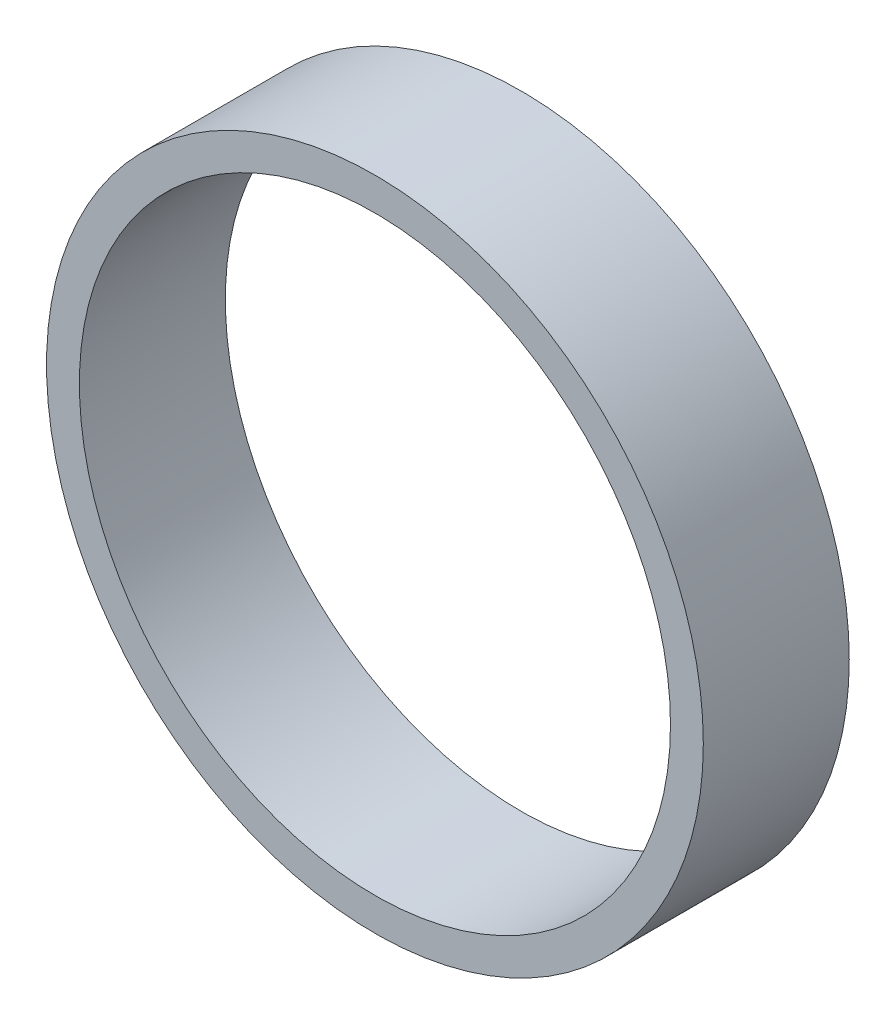
from build123d import *

# Parameters (mm, degrees)
SKETCH_1_R      = 22.5
SKETCH_1_R_2    = 20.25
EXTRUDE_1_DEPTH = 10


with BuildPart() as part:
    # 草图1 → 凸台-拉伸1 (new body)
    with BuildSketch(Plane.XY):
        Circle(SKETCH_1_R)
        Circle(SKETCH_1_R_2, mode=Mode.SUBTRACT)
    extrude(amount=EXTRUDE_1_DEPTH)


solid = part.part
